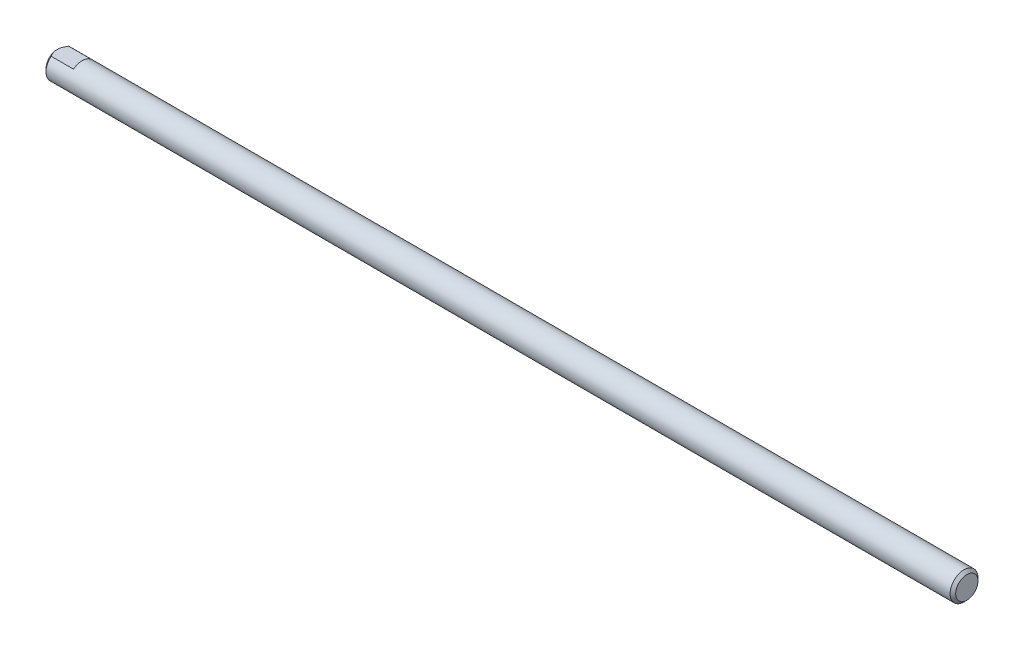
SolidWorks part; units mm, degrees
material "普通碳钢"
ref_plane "Front Plane" through (0, 0, 0) normal (0, 0, 1) x (1, 0, 0)
ref_plane "Top Plane" through (0, 0, 0) normal (0, 1, 0) x (1, 0, 0)
ref_plane "Right Plane" through (0, 0, 0) normal (1, 0, 0) x (0, 0, -1)
sketch "Sketch1" plane through (0, 0, 0) normal (1, 0, 0) x (0, 0, -1)
  circle A0 centre (0, 0) radius 5
  dimension "D1" = 10
extrude "Boss-Extrude1" add sketch "Sketch1" along normal blind 326
hole_wizard "M5 Tapped Hole1" positions "Sketch4" profile "Sketch5" tap size "M5" standard "GB"
sketch "Sketch4" plane through (0, 0, 0) normal (-1, 0, 0) x (0, 0, 1)
  point P0 (0, 0)
sketch "Sketch5" plane through (0, 0, 0) normal (0, 1, 0) x (0, 0, 1)
  line L0 (0, 0) -> (0, 13.6618)
  line L1 (0, 13.6618) -> (2.1, 12.4)
  line L2 (2.1, 12.4) -> (2.1, 0)
  line L5 (2.1, 0) -> (0, 0)
  line L10 (0, 13.6618) -> (-2.1, 12.4) construction
  line L11 (0, -6.35) -> (0, 107.95) construction
  dimension "螺纹孔钻头直径" = 4.2
  dimension "螺纹孔钻头深度" = 12.4
  dimension "导头角度" = 118
cosmetic thread "Cosmetic Thread 1" [suppressed] parameters "D1"=10, "D2"=5
hole_wizard "M5 Tapped Hole2" positions "Sketch6" profile "Sketch7" tap size "M5" standard "GB"
sketch "Sketch6" plane through (275, 0, 0) normal (1, 0, 0) x (0, 0, -1)
  point P0 (0, 0)
sketch "Sketch7" plane through (275, 0, 0) normal (0, 1, 0) x (0, 0, -1)
  line L0 (0, 0) -> (0, 13.6618)
  line L1 (0, 13.6618) -> (2.1, 12.4)
  line L2 (2.1, 12.4) -> (2.1, 0)
  line L5 (2.1, 0) -> (0, 0)
  line L10 (0, 13.6618) -> (-2.1, 12.4) construction
  line L11 (0, -6.35) -> (0, 107.95) construction
  dimension "螺纹孔钻头直径" = 4.2
  dimension "螺纹孔钻头深度" = 12.4
  dimension "导头角度" = 118
cosmetic thread "Cosmetic Thread 2" [suppressed] parameters "D1"=10, "D2"=5
chamfer "Chamfer1" distance 1 angle 45 2 edges at (0, 0, -5) (326, 0, -5)
sketch "Sketch8" plane through (0, 0, 0) normal (0, 0, 1) x (1, 0, 0)
  line L0 (326, 0) -> (271.6406, 0) construction
  line L1 (491.8129, 8.1428) -> (335, 8.1428)
  line L2 (491.8129, 8.1428) -> (491.8129, 3.9)
  line L3 (491.8129, 3.9) -> (335, 3.9)
  line L4 (335, 8.1428) -> (335, 3.9)
  line L5 (326, -5) -> (326, 5) construction
  line L6 (335, -8.1428) -> (335, -3.9)
  line L7 (491.8129, -3.9) -> (335, -3.9)
  line L8 (491.8129, -8.1428) -> (491.8129, -3.9)
  line L9 (491.8129, -8.1428) -> (335, -8.1428)
  line L10 (0, 0) -> (5.3658, 0) construction
  line L11 (-147.8129, 11.4756) -> (9, 11.4756)
  line L12 (-147.8129, 11.4756) -> (-147.8129, 3.9)
  line L13 (-147.8129, 3.9) -> (9, 3.9)
  line L14 (9, 11.4756) -> (9, 3.9)
  line L15 (9, -11.4756) -> (9, -3.9)
  line L16 (-147.8129, -3.9) -> (9, -3.9)
  line L17 (-147.8129, -11.4756) -> (-147.8129, -3.9)
  line L18 (-147.8129, -11.4756) -> (9, -11.4756)
  line L19 (0, 4) -> (0, -4) construction
  dimension "D1" = 7.8
  dimension "D2" = 9
  dimension "D3" = 7.8
  dimension "D4" = 9
extrude "Cut-Extrude1" cut sketch "Sketch8" against normal through all both and the other way through all
